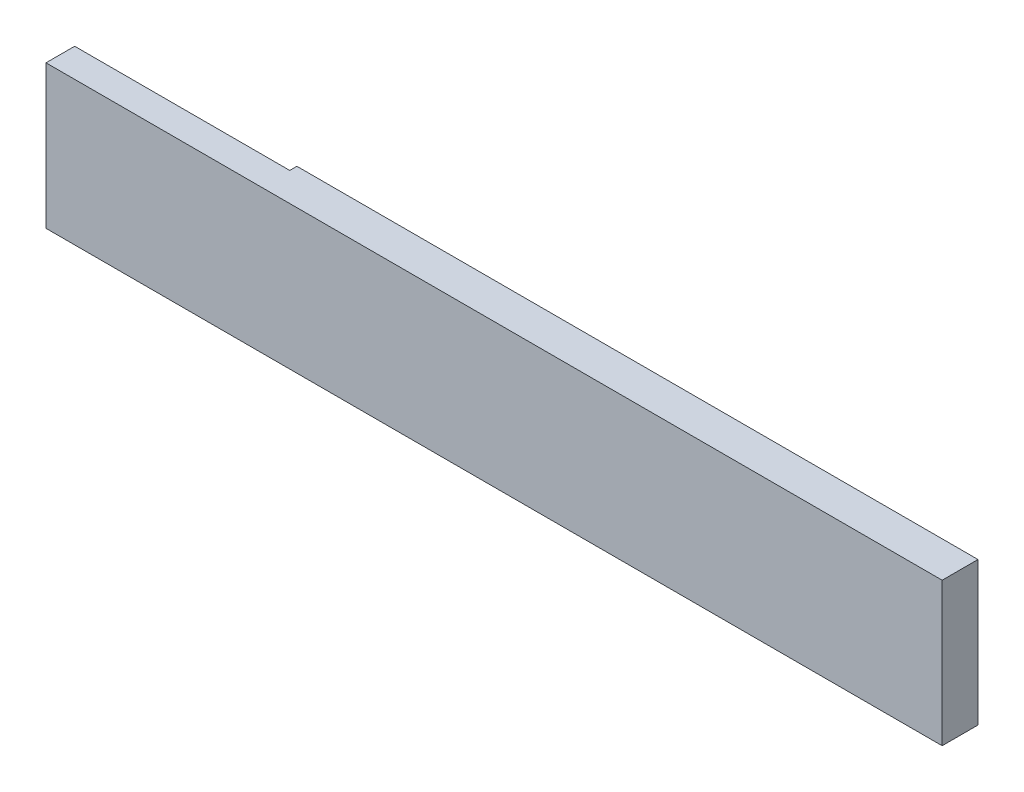
SolidWorks part; units mm, degrees
ref_plane "前视基准面" through (0, 0, 0) normal (0, 0, 1) x (1, 0, 0)
ref_plane "上视基准面" through (0, 0, 0) normal (0, 1, 0) x (1, 0, 0)
ref_plane "右视基准面" through (0, 0, 0) normal (1, 0, 0) x (0, 0, -1)
sketch "草图1" plane through (0, 0, 0) normal (0, 0, 1) x (1, 0, 0)
  line L1 (-125, -20) -> (125, -20)
  line L2 (-125, -20) -> (-125, 20)
  line L3 (-125, 20) -> (125, 20)
  line L4 (125, -20) -> (125, 20)
  line L5 (-125, -20) -> (125, 20) construction
  line L6 (-125, 20) -> (125, -20) construction
  point P0 (0, 0)
  dimension "D1" = 40
  dimension "D2" = 250
extrude "凸台-拉伸1" add sketch "草图1" along normal mid plane 10
sketch "草图2" plane through (0, 0, -5) normal (0, 0, -1) x (-1, 0, 0)
  line L0 (125, -20) -> (-125, -20) construction
  line L1 (125, 20) -> (65, 20)
  line L2 (125, 20) -> (125, -20)
  line L3 (125, -20) -> (65, -20)
  line L4 (65, 20) -> (65, -20)
  dimension "D1" = 60
extrude "切除-拉伸1" cut sketch "草图2" against normal blind 2
